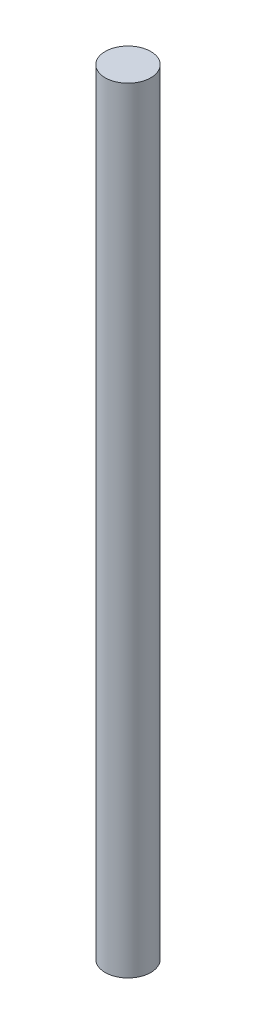
SolidWorks part; units mm, degrees
ref_plane "前视基准面" through (0, 0, 0) normal (0, 0, 1) x (1, 0, 0)
ref_plane "上视基准面" through (0, 0, 0) normal (0, 1, 0) x (1, 0, 0)
ref_plane "右视基准面" through (0, 0, 0) normal (1, 0, 0) x (0, 0, -1)
sketch "草图1" plane through (0, 0, 0) normal (0, 1, 0) x (1, 0, 0)
  circle A0 centre (0, 0) radius 1
  dimension "D1" = 2
extrude "凸台-拉伸1" add sketch "草图1" along normal blind 34
